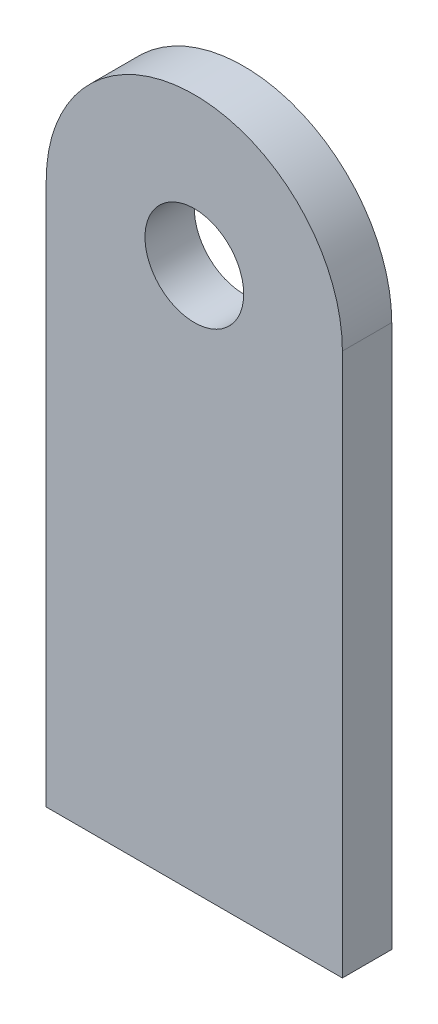
SolidWorks part; units mm, degrees
ref_plane "前视基准面" through (0, 0, 0) normal (0, 0, 1) x (1, 0, 0)
ref_plane "上视基准面" through (0, 0, 0) normal (0, 1, 0) x (1, 0, 0)
ref_plane "右视基准面" through (0, 0, 0) normal (1, 0, 0) x (0, 0, -1)
sketch "草图1" plane through (0, 0, 0) normal (0, 0, 1) x (1, 0, 0)
  line L0 (0, 0) -> (30, 0)
  line L3 (0, 0) -> (0, 55)
  line L4 (30, 0) -> (30, 55)
  circle A0 centre (15, 55) radius 5
  arc A1 (30, 55) -> (0, 55) centre (15, 55) ccw
extrude "凸台-拉伸1" add sketch "草图1" along normal blind 5
